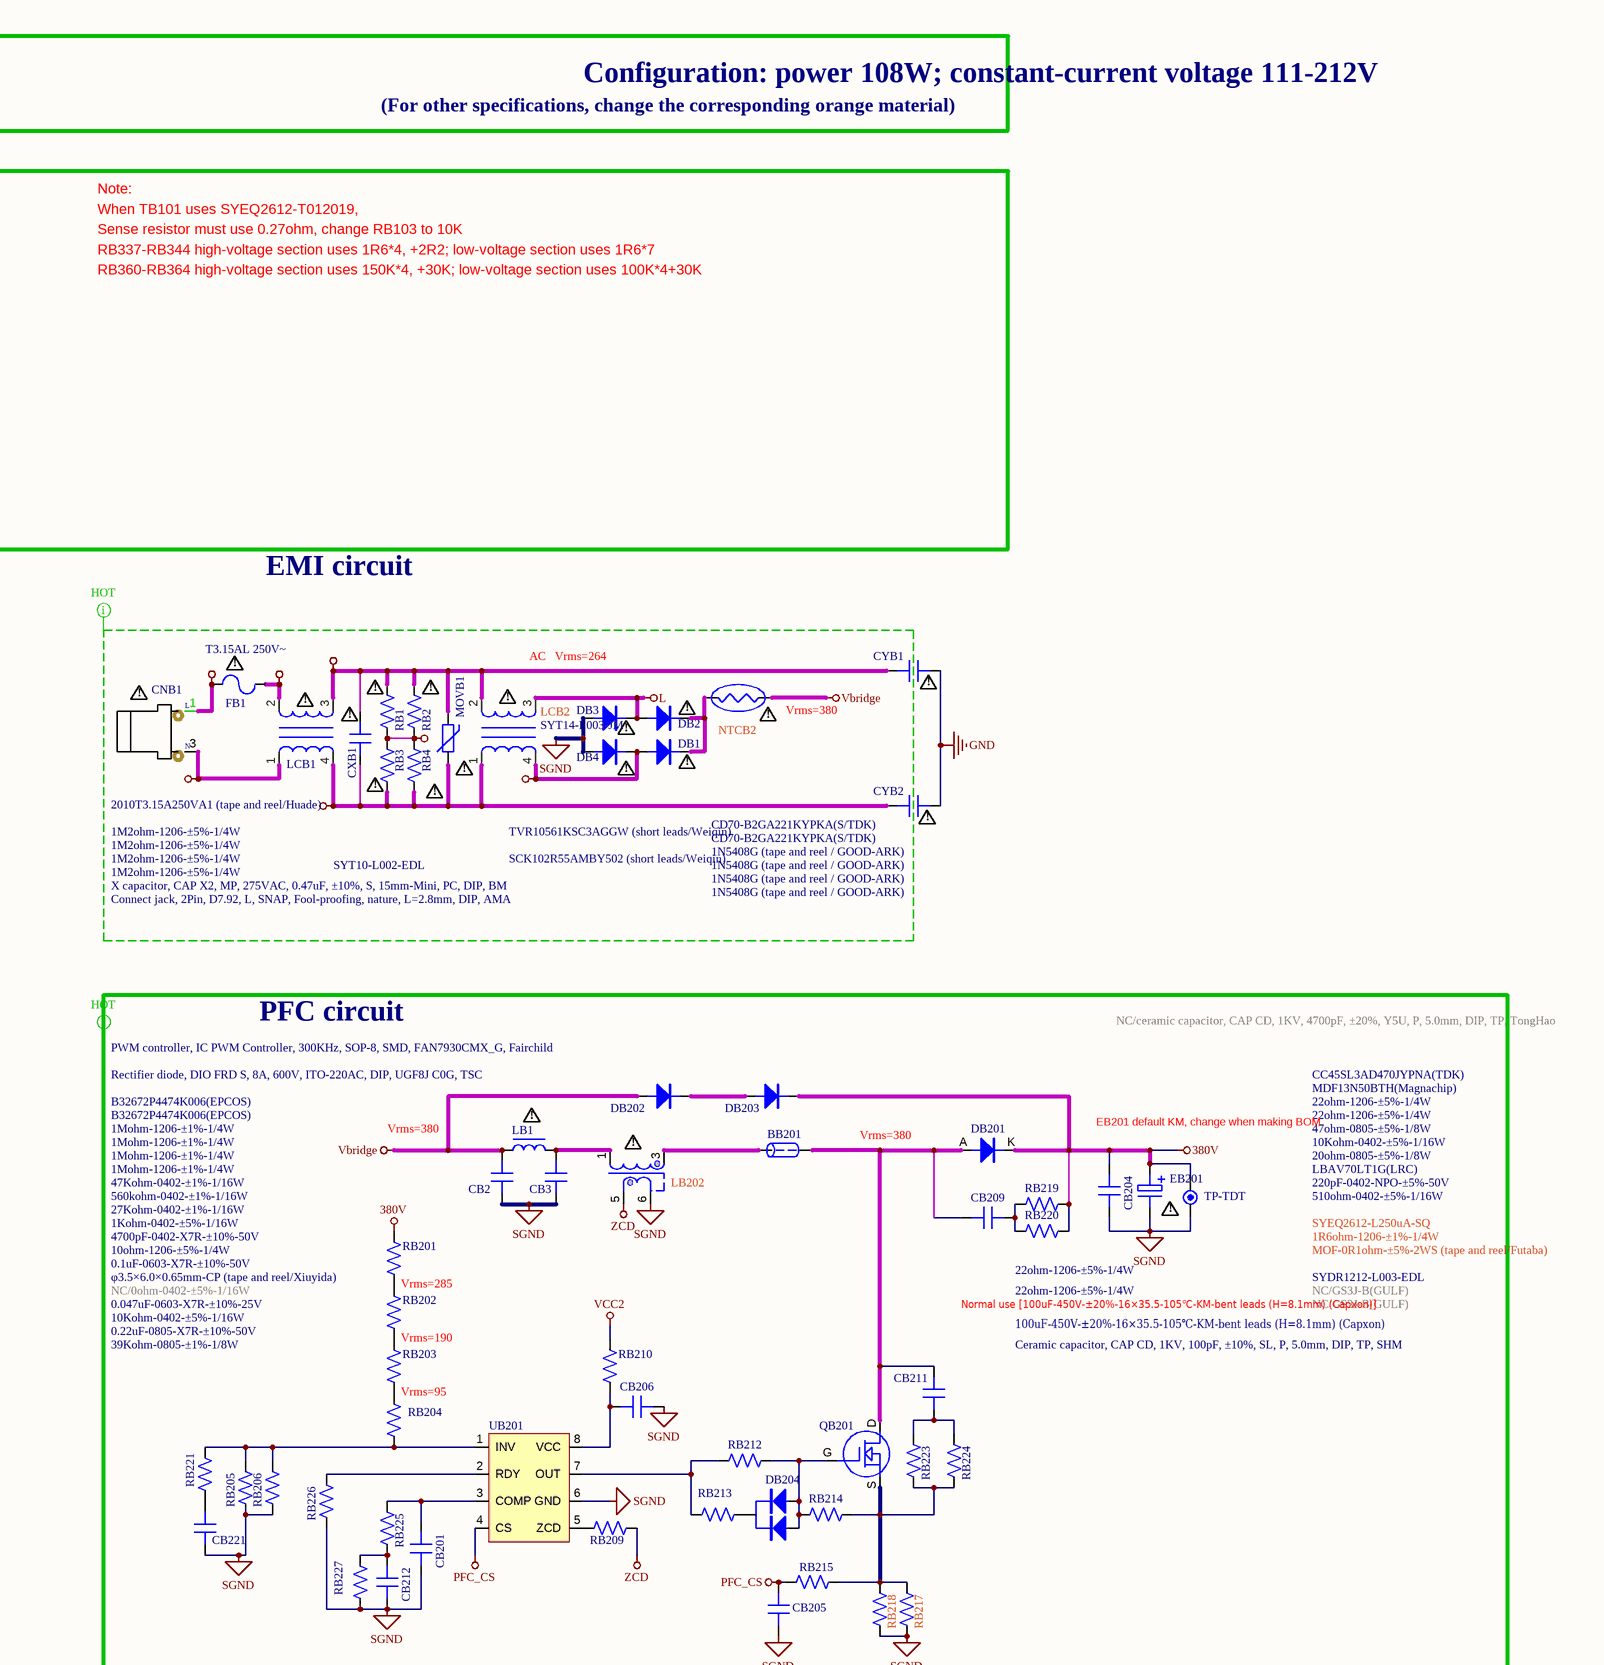
[diagram p0: PCBE84277.SchDoc, top left]
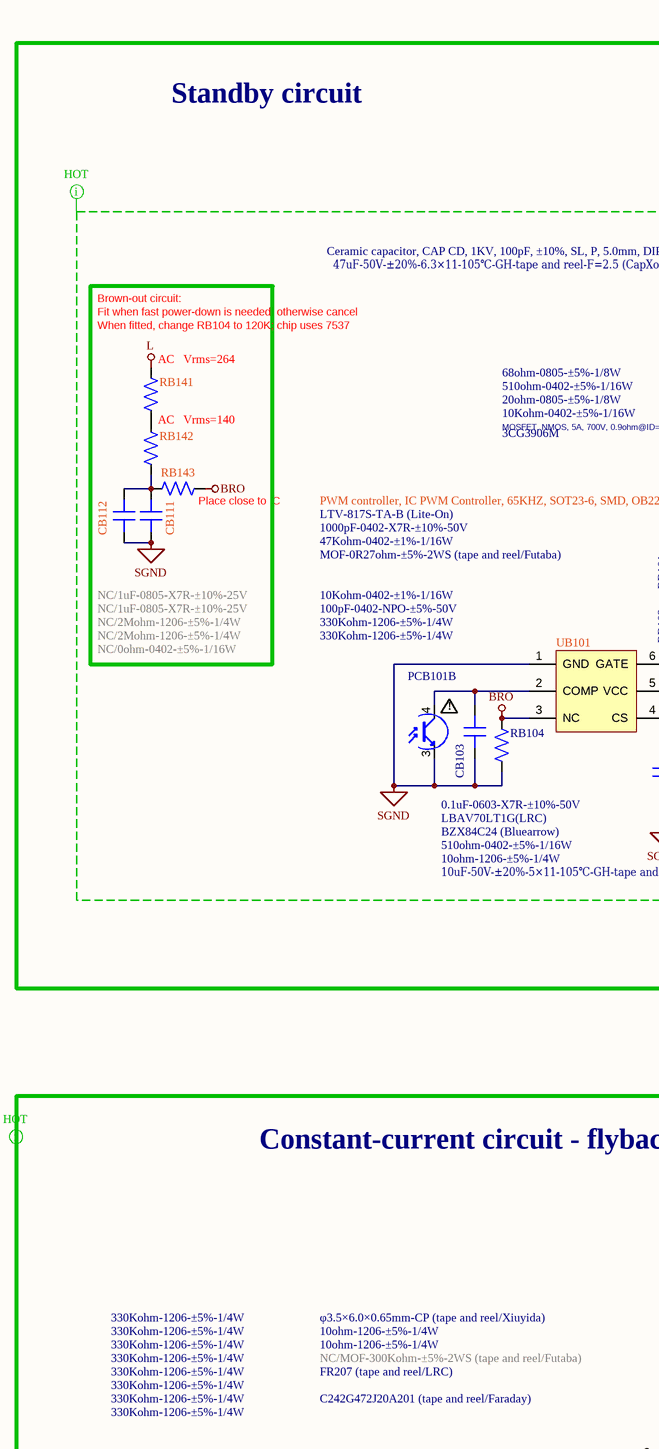
[diagram p1: PCBE84277.SchDoc, top middle]
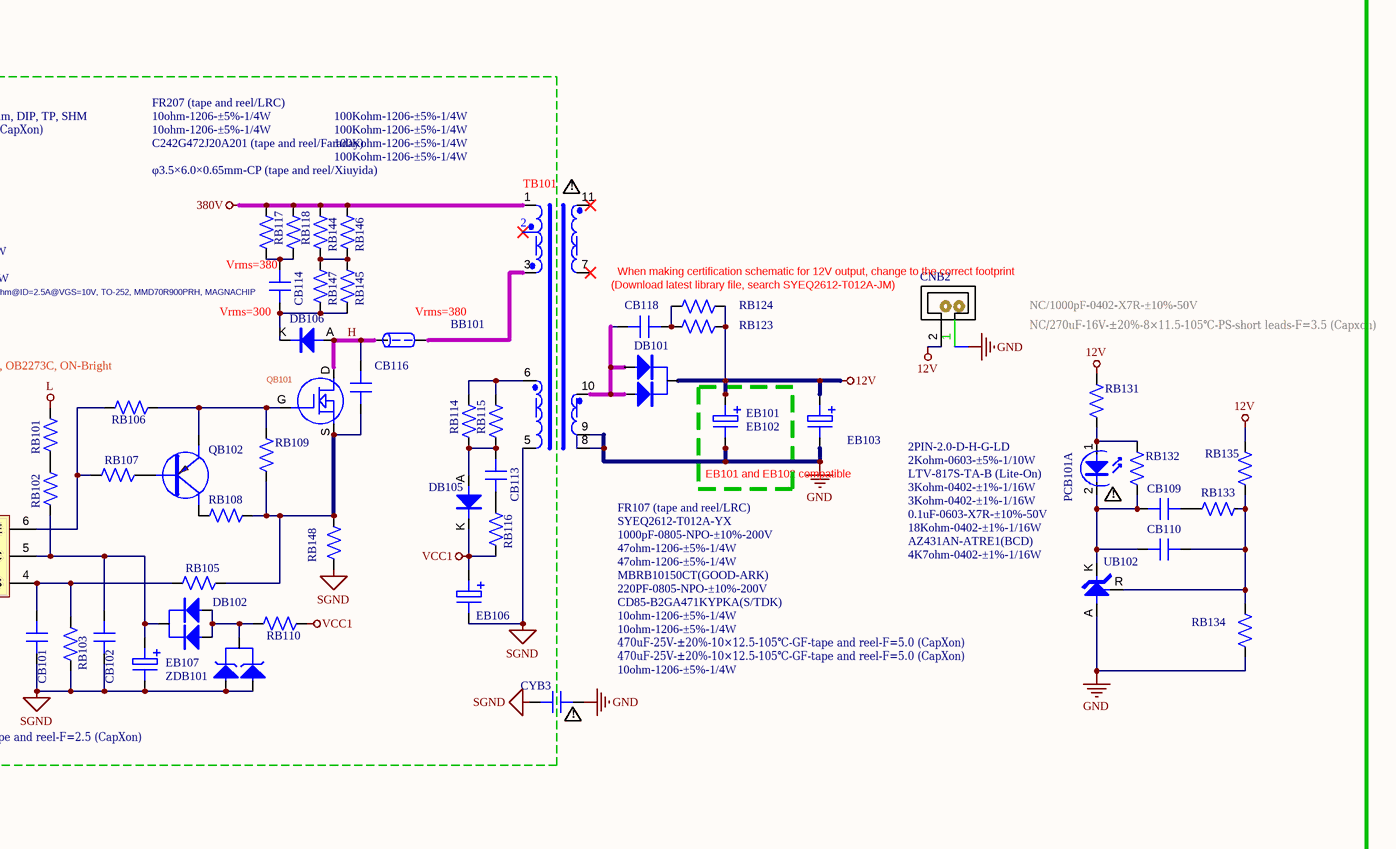
[diagram p2: PCBE84277.SchDoc, top right]
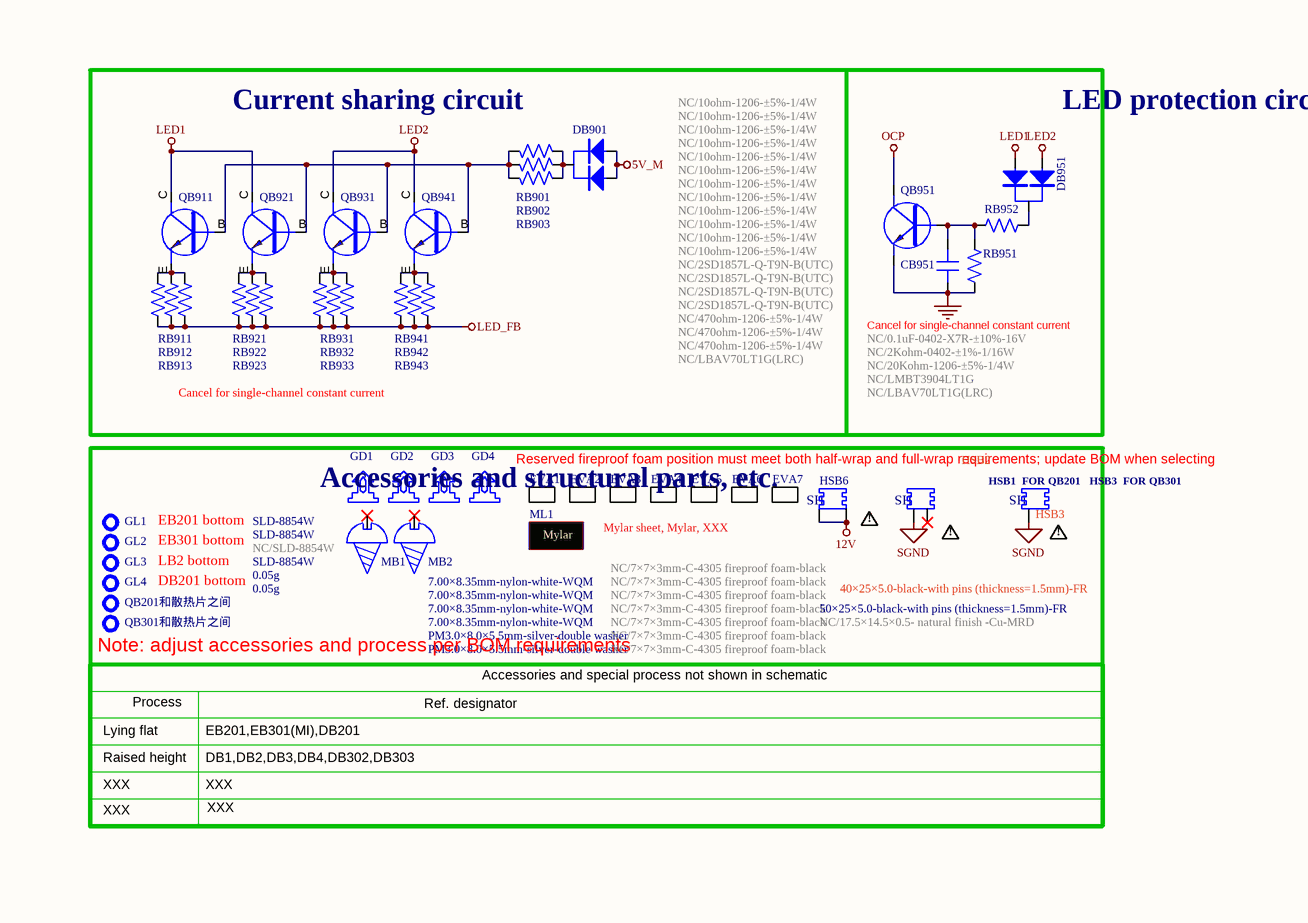
[diagram p3: PCBE84277.SchDoc, bottom left]
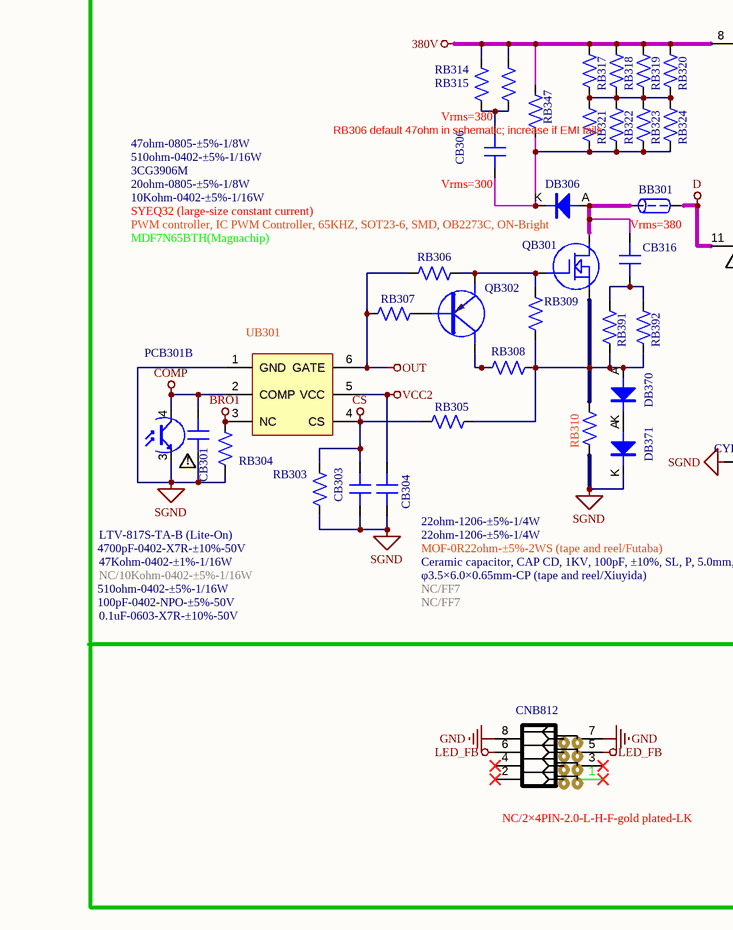
[diagram p4: PCBE84277.SchDoc, bottom middle]
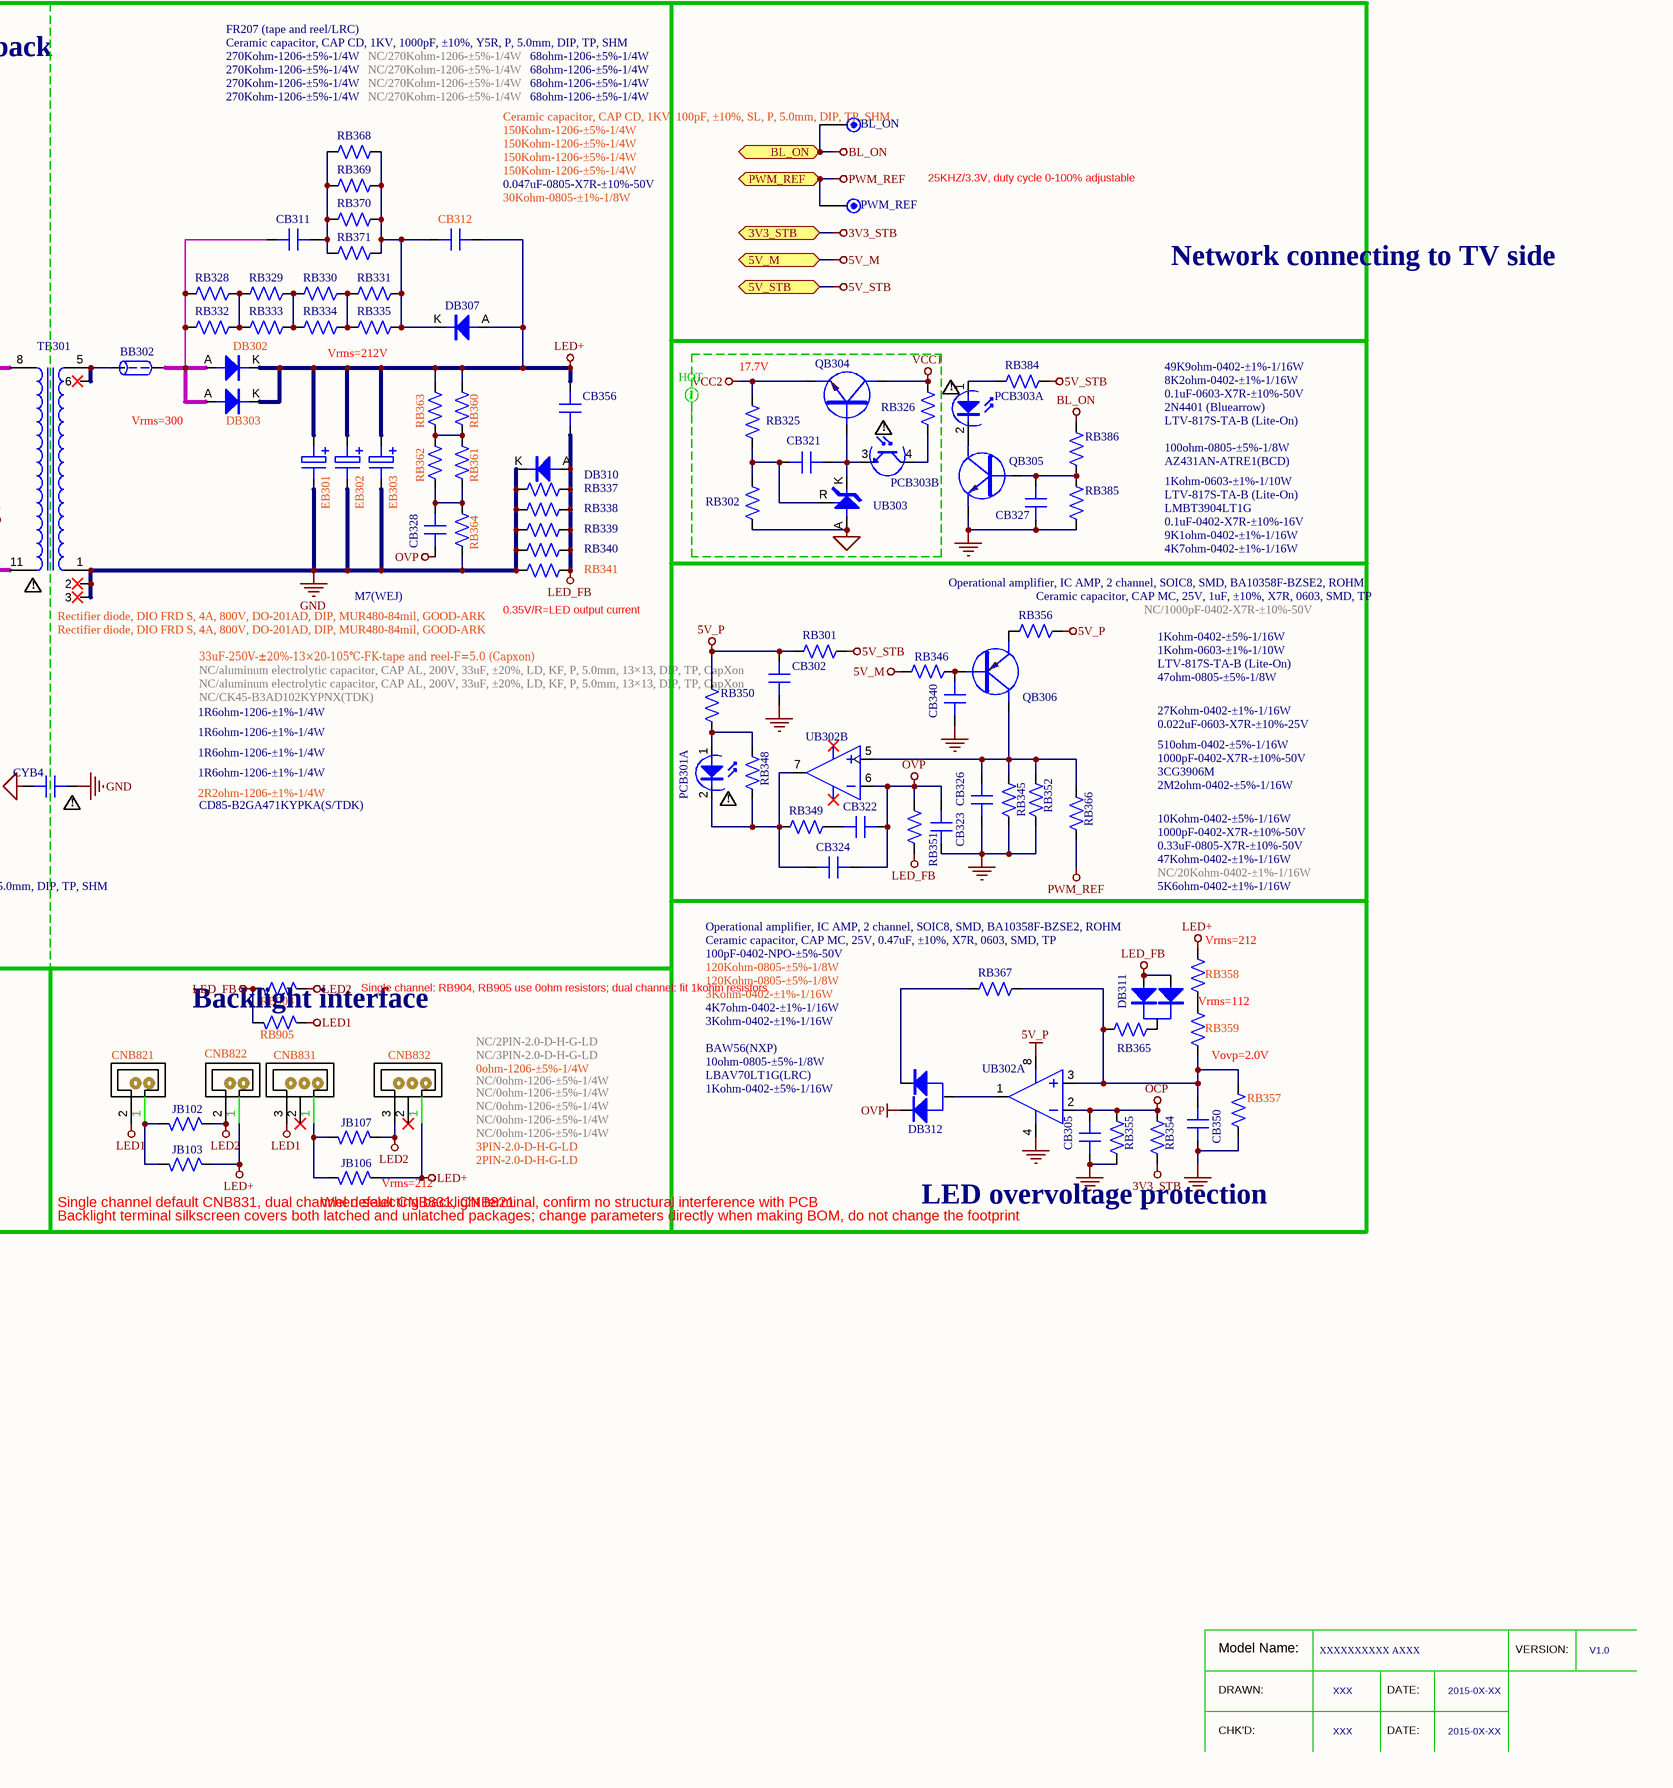
[diagram p5: PCBE84277.SchDoc, bottom right]
# Altium project MISC84277-14.PrjPCB (part 4 of 10)

## Sheet PCBE84277.SchDoc: MISC84277
size A1